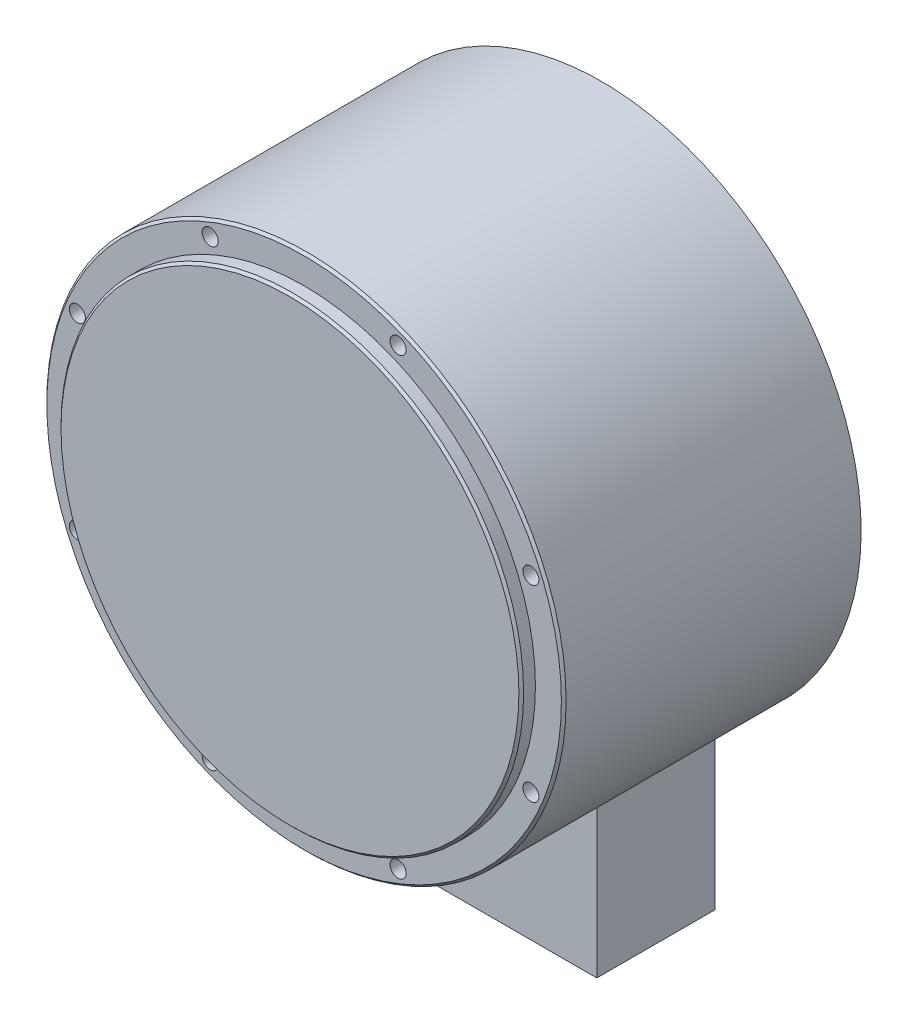
SolidWorks part; units mm, degrees
ref_plane "前视基准面" through (0, 0, 0) normal (0, 0, 1) x (1, 0, 0)
ref_plane "上视基准面" through (0, 0, 0) normal (0, 1, 0) x (1, 0, 0)
ref_plane "右视基准面" through (0, 0, 0) normal (1, 0, 0) x (0, 0, -1)
sketch "草图1" plane through (0, 0, 0) normal (0, 0, 1) x (1, 0, 0)
  circle A0 centre (0, 0) radius 110
  dimension "D1" = 220
extrude "凸台-拉伸1" add sketch "草图1" along normal blind 126
sketch "草图2" plane through (0, 0, 126) normal (0, 0, 1) x (1, 0, 0)
  circle A0 centre (0, 0) radius 98
  dimension "D1" = 196
extrude "凸台-拉伸2" add sketch "草图2" along normal blind 6
sketch "草图3" plane through (0, 0, 0) normal (0, 0, -1) x (-1, 0, 0)
  line L0 (0, 0) -> (0, -110) construction
  line L2 (-48, -98.9747) -> (48, -98.9747)
  line L3 (-48, -98.9747) -> (-48, -170)
  line L4 (-48, -170) -> (48, -170)
  line L5 (48, -98.9747) -> (48, -170)
  circle A0 centre (0, 0) radius 110 construction
  dimension "D1" = 96
  dimension "D2" = 280
extrude "凸台-拉伸3" add sketch "草图3" against normal blind 50
chamfer "倒角1" distance 1 angle 45 2 edges at (98, 0, 132) (110, 0, 126)
sketch "草图4" plane through (0, 0, 0) normal (0, 0, -1) x (-1, 0, 0)
  line L1 (-48, -170) -> (48, -170)
  line L2 (-48, -170) -> (-48, -74)
  line L3 (-48, -74) -> (48, -74)
  line L4 (48, -170) -> (48, -74)
extrude "凸台-拉伸4" [suppressed] add sketch "草图4" along normal blind 110 separate body
hole_wizard "M8 螺纹孔1" positions "草图5" profile "草图6" tap size "M8" standard "ISO"
sketch "草图5" plane through (0, 0, 0) normal (0, 0, -1) x (-1, 0, 0)
  line L0 (0, 0) -> (0, 115) construction
  line L2 (0, 0) -> (0, 115) construction
  point P0 (0, 115)
  point P11 (81.3173, 81.3173)
  point P12 (115, 0)
  point P13 (81.3173, -81.3173)
  point P14 (0, -115)
  point P15 (-81.3173, -81.3173)
  point P16 (-115, 0)
  point P17 (-81.3173, 81.3173)
  dimension "D1" = 115
  dimension "D2" = 8
sketch "草图6" plane through (0, 115, 0) normal (1, 0, 0) x (0, 1, 0)
  line L0 (0, 0) -> (0, 21.7929)
  line L1 (0, 21.7929) -> (3.4, 19.75)
  line L2 (3.4, 19.75) -> (3.4, 0)
  line L5 (3.4, 0) -> (0, 0)
  line L10 (0, 21.7929) -> (-3.4, 19.75) construction
  line L11 (0, -6.35) -> (0, 107.95) construction
  dimension "螺纹孔钻头直径" = 6.8
  dimension "螺纹孔钻头深度" = 19.75
  dimension "导头角度" = 118
cosmetic thread "孔螺蚊线4" parameters "D1"=16, "D2"=8
hole_wizard "M8 螺纹孔2" positions "草图7" profile "草图8" tap size "M8" standard "ISO"
sketch "草图7" plane through (0, 0, 132) normal (0, 0, 1) x (1, 0, 0)
  line L0 (0, 0) -> (39.7991, 96.0835) construction
  line L1 (0, 0) -> (0, 115.3677) construction
  point P34 (39.7991, 96.0835)
  point P40 (96.0835, 39.7991)
  point P41 (96.0835, -39.7991)
  point P42 (39.7991, -96.0835)
  point P43 (-39.7991, -96.0835)
  point P44 (-96.0835, -39.7991)
  point P45 (-96.0835, 39.7991)
  point P46 (-39.7991, 96.0835)
  dimension "D1" = 104
  dimension "D2" = 8
sketch "草图8" plane through (39.7991, 96.0835, 132) normal (1, 0, 0) x (0, -1, 0)
  line L0 (0, 0) -> (0, 21.7929)
  line L1 (0, 21.7929) -> (3.4, 19.75)
  line L2 (3.4, 19.75) -> (3.4, 0)
  line L5 (3.4, 0) -> (0, 0)
  line L10 (0, 21.7929) -> (-3.4, 19.75) construction
  line L11 (0, -6.35) -> (0, 107.95) construction
  dimension "螺纹孔钻头直径" = 6.8
  dimension "螺纹孔钻头深度" = 19.75
  dimension "导头角度" = 118
cosmetic thread "孔螺蚊线9" parameters "D1"=16, "D2"=8
cosmetic thread "孔螺蚊线10" parameters "D1"=16, "D2"=8
cosmetic thread "孔螺蚊线11" parameters "D1"=16, "D2"=8
cosmetic thread "孔螺蚊线12" parameters "D1"=16, "D2"=8
cosmetic thread "孔螺蚊线13" parameters "D1"=16, "D2"=8
cosmetic thread "孔螺蚊线14" parameters "D1"=16, "D2"=8
cosmetic thread "孔螺蚊线15" parameters "D1"=16, "D2"=8
cosmetic thread "孔螺蚊线16" parameters "D1"=16, "D2"=8
